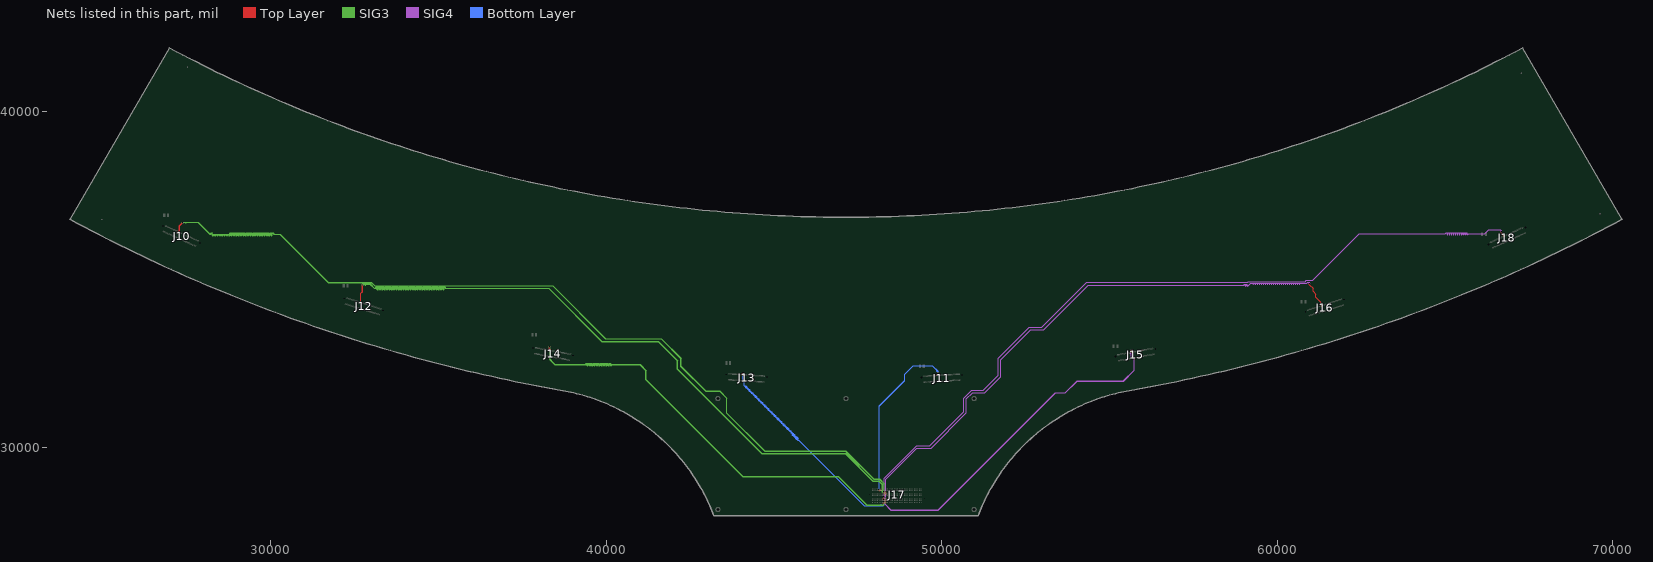
[diagram p0: the nets of this part, all layers, seen from the top]
# Altium PCB MISC86329.PcbDoc (part 8 of 11)
Units mil, origin at the board's own origin, x right, y up, seen from the top; angles counter-clockwise.
Board outline 46247.15 x 13937.21 mil, 6 copper layers (Top Layer, GND2, SIG3, SIG4, POWER5, Bottom Layer); 17 components, 210 nets, 908 pads, 1109 vias.

## Via types
v1: diameter 24, hole 12, Top Layer to Bottom Layer, 684 vias
v2: diameter 18, hole 9, Top Layer to Bottom Layer, 425 vias

## Nets (pads, with @x,y where several pads share a name; then routed paths per layer and width w, separated by ;. In a path a pad name is that pad's centre, name@x,y a point inside that pad or via, vN(x,y) a via of type N, cw(c..) or ccw(c..) an arc to the next point about the centre after c; other vN are vias at no path point) (continued)
DATAIN6N_CH0: J10.30 J17.G23 | length 28226.7
  Top Layer w5: J10.30@27279.03,36418.73 27279.03,36446.33 27291,36458.3 27291,36604 27383.75,36696.75 27386.6,36693.9 v2(27386.6,36690.4) ; v2(48264.09,28692.61) J17.G23@48287.89,28668.8
  SIG3 w5: v2@27383.75,36696.75 27398,36711 27462,36711 27467,36706 27467,36697.6 27472,36692.6 27482,36692.6 27487,36697.6 27487,36706 27492,36711 27838,36711 28196,36353 28223.82,36353 28235.5,36364.68 28235.5,36386.58 28241.32,36392.41 28254.68,36392.41 28260.5,36386.58 28260.5,36325.27 28272.18,36313.59 28293.82,36313.59 28305.5,36325.27 28305.5,36347.18 28311.32,36353 28324.68,36353 28330.5,36347.18 28330.5,36325.27 28342.18,36313.59 28363.82,36313.59 28375.5,36325.27 28375.5,36347.18 28381.32,36353 28394.68,36353 28400.5,36347.18 28400.5,36325.27 28412.18,36313.59 28433.82,36313.59 28445.5,36325.27 28445.5,36347.18 28451.32,36353 28464.68,36353 28470.5,36347.18 28470.5,36325.27 28482.18,36313.59 28503.82,36313.59 28515.5,36325.27 28515.5,36347.18 28521.32,36353 28534.68,36353 28540.5,36347.18 28540.5,36325.27 28552.18,36313.59 28573.82,36313.59 28585.5,36325.27 28585.5,36347.18 28591.32,36353 28604.68,36353 28610.5,36347.18 28610.5,36325.27 28622.18,36313.59 28643.82,36313.59 28655.5,36325.27 28655.5,36347.18 28661.32,36353 28674.68,36353 28680.5,36347.18 28680.5,36325.27 28692.18,36313.59 28713.82,36313.59 28725.5,36325.27 28725.5,36347.18 28731.32,36353 28744.68,36353 28750.5,36347.18 28750.5,36325.27 28762.18,36313.59 28783.82,36313.59 28795.5,36325.27 28795.5,36386.58 28801.32,36392.41 28814.68,36392.41 28820.5,36386.58 28820.5,36325.27 28832.18,36313.59 28853.82,36313.59 28865.5,36325.27 28865.5,36386.58 28871.32,36392.41 28884.68,36392.41 28890.5,36386.58 28890.5,36325.27 28902.18,36313.59 28923.82,36313.59 28935.5,36325.27 28935.5,36386.58 28941.32,36392.41 28954.68,36392.41 28960.5,36386.58 28960.5,36325.27 28972.18,36313.59 28993.82,36313.59 29005.5,36325.27 29005.5,36386.58 29011.32,36392.41 29024.68,36392.41 29030.5,36386.58 29030.5,36325.27 29042.18,36313.59 29063.82,36313.59 29075.5,36325.27 29075.5,36386.58 29081.32,36392.41 29094.68,36392.41 29100.5,36386.58 29100.5,36325.27 29112.18,36313.59 29133.82,36313.59 29145.5,36325.27 29145.5,36386.58 29151.32,36392.41 29164.68,36392.41 29170.5,36386.58 29170.5,36325.27 29182.18,36313.59 29203.82,36313.59 29215.5,36325.27 29215.5,36386.58 29221.32,36392.41 29234.68,36392.41 29240.5,36386.58 29240.5,36325.27 29252.18,36313.59 29273.82,36313.59 29285.5,36325.27 29285.5,36386.58 29291.32,36392.41 29304.68,36392.41 29310.5,36386.58 29310.5,36325.27 29322.18,36313.59 29343.82,36313.59 29355.5,36325.27 29355.5,36386.58 29361.32,36392.41 29374.68,36392.41 29380.5,36386.58 29380.5,36325.27 29392.18,36313.59 29413.82,36313.59 29425.5,36325.27 29425.5,36386.58 29431.32,36392.41 29444.68,36392.41 29450.5,36386.58 29450.5,36325.27 29462.18,36313.59 29483.82,36313.59 29495.5,36325.27 29495.5,36386.58 29501.32,36392.41 29514.68,36392.41 29520.5,36386.58 29520.5,36325.27 29532.18,36313.59 29553.82,36313.59 29565.5,36325.27 29565.5,36386.58 29571.32,36392.41 29584.68,36392.41 29590.5,36386.58 29590.5,36325.27 29602.18,36313.59 29623.82,36313.59 29635.5,36325.27 29635.5,36386.58 29641.32,36392.41 29654.68,36392.41 29660.5,36386.58 29660.5,36325.27 29672.18,36313.59 29693.82,36313.59 29705.5,36325.27 29705.5,36386.58 29711.32,36392.41 29724.68,36392.41 29730.5,36386.58 29730.5,36325.27 29742.18,36313.59 29763.82,36313.59 29775.5,36325.27 29775.5,36386.58 29781.32,36392.41 29794.68,36392.41 29800.5,36386.58 29800.5,36325.27 29812.18,36313.59 29833.82,36313.59 29845.5,36325.27 29845.5,36386.58 29851.32,36392.41 29864.68,36392.41 29870.5,36386.58 29870.5,36325.27 29882.18,36313.59 29903.82,36313.59 29915.5,36325.27 29915.5,36386.58 29921.32,36392.41 29934.68,36392.41 29940.5,36386.58 29940.5,36325.27 29952.18,36313.59 29973.82,36313.59 29985.5,36325.27 29985.5,36386.58 29991.32,36392.41 30004.68,36392.41 30010.5,36386.58 30010.5,36325.27 30022.18,36313.59 30043.82,36313.59 30055.5,36325.27 30055.5,36386.58 30061.32,36392.41 30074.68,36392.41 30080.5,36386.58 30080.5,36364.68 30092.18,36353 30281.86,36353 31717.86,34917 33003.86,34917 33104.86,34816 38404.86,34816 39981.86,33239 41642,33239 42230,32651 42230,32414.86 42966.86,31678 43382.86,31678 43592,31468.86 43592,31025.86 44721.86,29896 47133.86,29896 47970.86,29059 48145.86,29059 48284.09,28920.77 48284.09,28712.61 v2(48264.09,28692.61)
DATAIN6N_CH1: J12.30 J17.F23 | length 23094.8
  Top Layer w5: J12.30@32696.65,34319.49 32696,34320.14 32696,34596 32745,34645 32745,34837.5 v2(32751.5,34844) ; v2(48264.09,28642.61) J17.F23@48287.89,28618.8
  SIG3 w5: v2(32751.5,34844) 32745,34850.5 32745,34857.86 32756.14,34869 32783,34869 32795.5,34869 32814.25,34869 32820.5,34862.75 32820.5,34838.79 32826.75,34832.54 32839.25,34832.54 32845.5,34838.79 32845.5,34862.75 32851.75,34869 32962,34869 32970.84,34860.16 ; 32964.5,34866.5 33089,34742 33134.82,34742 33146.5,34753.68 33146.5,34775.69 33152.32,34781.52 33165.68,34781.52 33171.5,34775.69 33171.5,34714.16 33183.18,34702.48 33204.82,34702.48 33216.5,34714.16 33216.5,34775.69 33222.32,34781.52 33235.68,34781.52 33241.5,34775.69 33241.5,34714.16 33253.18,34702.48 33274.82,34702.48 33286.5,34714.16 33286.5,34775.69 33292.32,34781.52 33305.68,34781.52 33311.5,34775.69 33311.5,34714.16 33323.18,34702.48 33344.82,34702.48 33356.5,34714.16 33356.5,34775.69 33362.32,34781.52 33375.68,34781.52 33381.5,34775.69 33381.5,34714.16 33393.18,34702.48 33414.82,34702.48 33426.5,34714.16 33426.5,34775.69 33432.32,34781.52 33445.68,34781.52 33451.5,34775.69 33451.5,34714.16 33463.18,34702.48 33484.82,34702.48 33496.5,34714.16 33496.5,34775.69 33502.32,34781.52 33515.68,34781.52 33521.5,34775.69 33521.5,34714.16 33533.18,34702.48 33554.82,34702.48 33566.5,34714.16 33566.5,34775.69 33572.32,34781.52 33585.68,34781.52 33591.5,34775.69 33591.5,34714.16 33603.18,34702.48 33624.82,34702.48 33636.5,34714.16 33636.5,34775.69 33642.32,34781.52 33655.68,34781.52 33661.5,34775.69 33661.5,34714.16 33673.18,34702.48 33694.82,34702.48 33706.5,34714.16 33706.5,34775.69 33712.32,34781.52 33725.68,34781.52 33731.5,34775.69 33731.5,34714.16 33743.18,34702.48 33764.82,34702.48 33776.5,34714.16 33776.5,34775.69 33782.32,34781.52 33795.68,34781.52 33801.5,34775.69 33801.5,34714.16 33813.18,34702.48 33834.82,34702.48 33846.5,34714.16 33846.5,34775.69 33852.32,34781.52 33865.68,34781.52 33871.5,34775.69 33871.5,34714.16 33883.18,34702.48 33904.82,34702.48 33916.5,34714.16 33916.5,34775.69 33922.32,34781.52 33935.68,34781.52 33941.5,34775.69 33941.5,34714.16 33953.18,34702.48 33974.82,34702.48 33986.5,34714.16 33986.5,34775.69 33992.32,34781.52 34005.68,34781.52 34011.5,34775.69 34011.5,34714.16 34023.18,34702.48 34044.82,34702.48 34056.5,34714.16 34056.5,34775.69 34062.32,34781.52 34075.68,34781.52 34081.5,34775.69 34081.5,34714.16 34093.18,34702.48 34114.82,34702.48 34126.5,34714.16 34126.5,34775.69 34132.32,34781.52 34145.68,34781.52 34151.5,34775.69 34151.5,34714.16 34163.18,34702.48 34184.82,34702.48 34196.5,34714.16 34196.5,34775.69 34202.32,34781.52 34215.68,34781.52 34221.5,34775.69 34221.5,34714.16 34233.18,34702.48 34254.82,34702.48 34266.5,34714.16 34266.5,34775.69 34272.32,34781.52 34285.68,34781.52 34291.5,34775.69 34291.5,34714.16 34303.18,34702.48 34324.82,34702.48 34336.5,34714.16 34336.5,34775.69 34342.32,34781.52 34355.68,34781.52 34361.5,34775.69 34361.5,34714.16 34373.18,34702.48 34394.82,34702.48 34406.5,34714.16 34406.5,34775.69 34412.32,34781.52 34425.68,34781.52 34431.5,34775.69 34431.5,34714.16 34443.18,34702.48 34464.82,34702.48 34476.5,34714.16 34476.5,34775.69 34482.32,34781.52 34495.68,34781.52 34501.5,34775.69 34501.5,34714.16 34513.18,34702.48 34534.82,34702.48 34546.5,34714.16 34546.5,34775.69 34552.32,34781.52 34565.68,34781.52 34571.5,34775.69 34571.5,34714.16 34583.18,34702.48 34604.82,34702.48 34616.5,34714.16 34616.5,34775.69 34622.32,34781.52 34635.68,34781.52 34641.5,34775.69 34641.5,34714.16 34653.18,34702.48 34674.82,34702.48 34686.5,34714.16 34686.5,34775.69 34692.32,34781.52 34705.68,34781.52 34711.5,34775.69 34711.5,34714.16 34723.18,34702.48 34744.82,34702.48 34756.5,34714.16 34756.5,34775.69 34762.32,34781.52 34775.68,34781.52 34781.5,34775.69 34781.5,34714.16 34793.18,34702.48 34814.82,34702.48 34826.5,34714.16 34826.5,34775.69 34832.32,34781.52 34845.68,34781.52 34851.5,34775.69 34851.5,34714.16 34863.18,34702.48 34884.82,34702.48 34896.5,34714.16 34896.5,34775.69 34902.32,34781.52 34915.68,34781.52 34921.5,34775.69 34921.5,34714.16 34933.18,34702.48 34954.82,34702.48 34966.5,34714.16 34966.5,34775.69 34972.32,34781.52 34985.68,34781.52 34991.5,34775.69 34991.5,34714.16 35003.18,34702.48 35024.82,34702.48 35036.5,34714.16 35036.5,34775.69 35042.32,34781.52 35055.68,34781.52 35061.5,34775.69 35061.5,34714.16 35073.18,34702.48 35094.82,34702.48 35106.5,34714.16 35106.5,34775.69 35112.32,34781.52 35125.68,34781.52 35131.5,34775.69 35131.5,34714.16 35143.18,34702.48 35164.82,34702.48 35176.5,34714.16 35176.5,34775.69 35182.32,34781.52 35195.68,34781.52 35201.5,34775.69 35201.5,34753.68 35213.18,34742 38287.86,34742 39873.86,33156 41550,33156 42119,32587 42119,32333.86 44637.86,29815 47132.86,29815 47944.86,29003 48126.86,29003 48233,28896.86 48233,28676 48256.96,28652.04 48264.09,28644.91 v2(48264.09,28642.61)
DATAIN6N_CH2: J14.30 J17.B23 | length 13805.7
  Top Layer w5: v2(38324.5,33005) 38318,32998.5 38318,32928 38329.73,32916.27 J14.30@38329.73,32896.14 ; v2(48264.09,28395) J17.B23@48287.89,28418.8
  SIG3 w5: v2@38322,33002 38317,32997 38317,32962.14 38330,32949.14 38330,32898.75 38336.25,32892.5 38343.96,32892.5 38350.21,32886.25 38350.21,32873.75 38343.96,32867.5 38336.25,32867.5 38330,32861.25 38330,32629 38347.49,32611.51 38361.25,32597.75 38381.81,32577.19 38476,32483 39384.68,32483 39390.5,32488.82 39390.5,32501.32 39402.18,32513 39423.82,32513 39435.5,32501.32 39435.5,32451.39 39441.32,32445.57 39454.68,32445.57 39460.5,32451.39 39460.5,32501.32 39472.18,32513 39493.82,32513 39505.5,32501.32 39505.5,32451.39 39511.32,32445.57 39524.68,32445.57 39530.5,32451.39 39530.5,32501.32 39542.18,32513 39563.82,32513 39575.5,32501.32 39575.5,32451.39 39581.32,32445.57 39594.68,32445.57 39600.5,32451.39 39600.5,32501.32 39612.18,32513 39633.82,32513 39645.5,32501.32 39645.5,32451.39 39651.32,32445.57 39664.68,32445.57 39670.5,32451.39 39670.5,32501.32 39682.18,32513 39703.82,32513 39715.5,32501.32 39715.5,32451.39 39721.32,32445.57 39734.68,32445.57 39740.5,32451.39 39740.5,32501.32 39752.18,32513 39773.82,32513 39785.5,32501.32 39785.5,32451.39 39791.32,32445.57 39804.68,32445.57 39810.5,32451.39 39810.5,32501.32 39822.18,32513 39843.82,32513 39855.5,32501.32 39855.5,32451.39 39861.32,32445.57 39874.68,32445.57 39880.5,32451.39 39880.5,32501.32 39892.18,32513 39913.82,32513 39925.5,32501.32 39925.5,32451.39 39931.32,32445.57 39944.68,32445.57 39950.5,32451.39 39950.5,32501.32 39962.18,32513 39983.82,32513 39995.5,32501.32 39995.5,32451.39 40001.32,32445.57 40014.68,32445.57 40020.5,32451.39 40020.5,32501.32 40032.18,32513 40053.82,32513 40065.5,32501.32 40065.5,32451.39 40071.32,32445.57 40084.68,32445.57 40090.5,32451.39 40090.5,32501.32 40102.18,32513 40123.82,32513 40135.5,32501.32 40135.5,32451.39 40141.32,32445.57 40154.68,32445.57 40160.5,32451.39 40160.5,32471.32 40172.18,32483 41011,32483 41199,32295 41199,32024 44075,29148 46915,29148 47770,28293 48253,28293 48285,28325 48285,28374.09 v2(48264.09,28395)
DATAIN6N_CH3: J13.30 J17.A23 | length 7746.4
  Top Layer w5: 44083.13,32206.15 44094.28,32195 J13.30@44094.28,32169.89 ; 44083.56,32206.58 44083.56,32233.5 ; v2(48264.09,28345) J17.A23@48287.89,28368.8
  Bottom Layer w5: 44084,32223 44084,32222 ; v2(44090.06,32240) 44084,32233.94 44084,32222 ; v2(48264.09,28345) 48284.09,28325 48284.09,28300 48254.09,28270 48213.82,28270 48210.5,28273.32 48210.5,28280.82 48201.32,28290 48184.68,28290 48175.5,28280.82 48175.5,28273.32 48172.18,28270 47699.14,28270 45732.97,30236.17 45721.76,30236.17 45714.69,30229.1 45711.76,30229.1 45704.08,30236.78 45704.08,30239.71 45725.29,30260.92 45725.29,30272.13 45711.76,30285.67 45700.54,30285.67 45679.33,30264.46 45676.4,30264.46 45668.72,30272.13 45668.72,30275.06 45689.94,30296.27 45689.94,30307.49 45676.4,30321.02 45665.19,30321.02 45643.98,30299.81 45641.05,30299.81 45633.37,30307.49 45633.37,30310.42 45654.58,30331.63 45654.58,30342.84 45641.05,30356.38 45629.83,30356.38 45608.62,30335.17 45605.69,30335.17 45598.01,30342.84 45598.01,30345.77 45619.23,30366.99 45619.23,30378.2 45605.69,30391.73 45594.48,30391.73 45573.27,30370.52 45570.34,30370.52 45562.66,30378.2 45562.66,30381.13 45583.87,30402.34 45583.87,30413.55 45570.34,30427.09 45559.12,30427.09 45552.05,30420.02 45549.12,30420.02 45541.45,30427.7 45541.45,30430.63 45548.52,30437.7 45548.52,30448.91 45534.98,30462.44 45523.77,30462.44 45516.7,30455.37 45513.77,30455.37 45506.09,30463.05 45506.09,30465.98 45513.16,30473.05 45513.16,30484.26 45499.63,30497.8 45488.41,30497.8 45481.34,30490.73 45478.41,30490.73 45470.74,30498.41 45470.74,30501.34 45477.81,30508.41 45477.81,30519.62 45464.27,30533.16 45453.06,30533.16 45445.99,30526.08 45443.06,30526.08 45435.38,30533.76 45435.38,30536.69 45442.45,30543.76 45442.45,30554.98 45428.92,30568.51 45417.7,30568.51 45410.63,30561.44 45407.7,30561.44 45400.02,30569.12 45400.02,30572.05 45407.1,30579.12 45407.1,30590.33 45393.56,30603.87 45382.35,30603.87 45375.28,30596.8 45372.35,30596.8 45364.67,30604.47 45364.67,30607.4 45371.74,30614.47 45371.74,30625.69 45358.2,30639.22 45346.99,30639.22 45339.92,30632.15 45336.99,30632.15 45329.31,30639.83 45329.31,30642.76 45336.38,30649.83 45336.38,30661.04 45322.85,30674.58 45311.64,30674.58 45304.56,30667.51 45301.64,30667.51 45293.96,30675.18 45293.96,30678.11 45301.03,30685.18 45301.03,30696.4 45287.49,30709.93 45276.28,30709.93 45269.21,30702.86 45266.28,30702.86 45258.6,30710.54 45258.6,30713.47 45265.67,30720.54 45265.67,30731.75 45252.14,30745.29 45240.93,30745.29 45233.85,30738.22 45230.93,30738.22 45223.25,30745.89 45223.25,30748.82 45230.32,30755.89 45230.32,30767.11 45216.78,30780.64 45205.57,30780.64 45198.5,30773.57 45195.57,30773.57 45187.89,30781.25 45187.89,30784.18 45194.96,30791.25 45194.96,30802.46 45181.43,30816 45170.21,30816 45163.14,30808.93 45160.21,30808.93 45152.54,30816.6 45152.54,30819.53 45159.61,30826.6 45159.61,30837.82 45146.07,30851.35 45134.86,30851.35 45127.79,30844.28 45124.86,30844.28 45117.18,30851.96 45117.18,30854.89 45124.25,30861.96 45124.25,30873.17 45110.72,30886.71 45099.5,30886.71 45092.43,30879.64 45089.5,30879.64 45081.83,30887.32 45081.83,30890.24 45088.9,30897.32 45088.9,30908.53 45075.36,30922.06 45064.15,30922.06 45057.08,30914.99 45054.15,30914.99 45046.47,30922.67 45046.47,30925.6 45053.54,30932.67 45053.54,30943.88 45040.01,30957.42 45028.79,30957.42 45021.72,30950.35 45018.79,30950.35 45011.12,30958.03 45011.12,30960.96 45018.19,30968.03 45018.19,30979.24 45004.65,30992.78 44993.44,30992.78 44986.37,30985.7 44983.44,30985.7 44975.76,30993.38 44975.76,30996.31 44982.83,31003.38 44982.83,31014.6 44969.3,31028.13 44958.08,31028.13 44951.01,31021.06 44948.08,31021.06 44940.4,31028.74 44940.4,31031.67 44947.48,31038.74 44947.48,31049.95 44933.94,31063.49 44922.73,31063.49 44915.66,31056.41 44912.73,31056.41 44905.05,31064.09 44905.05,31067.02 44912.12,31074.09 44912.12,31085.31 44898.59,31098.84 44887.37,31098.84 44880.3,31091.77 44877.37,31091.77 44869.69,31099.45 44869.69,31102.38 44876.77,31109.45 44876.77,31120.66 44863.23,31134.2 44852.02,31134.2 44844.95,31127.13 44842.02,31127.13 44834.34,31134.8 44834.34,31137.73 44841.41,31144.8 44841.41,31156.02 44827.87,31169.55 44816.66,31169.55 44809.59,31162.48 44806.66,31162.48 44798.98,31170.16 44798.98,31173.09 44806.05,31180.16 44806.05,31191.37 44792.52,31204.91 44781.31,31204.91 44774.23,31197.84 44771.31,31197.84 44763.63,31205.51 44763.63,31208.44 44770.7,31215.51 44770.7,31226.73 44757.16,31240.26 44745.95,31240.26 44738.88,31233.19 44735.95,31233.19 44728.27,31240.87 44728.27,31243.8 44735.34,31250.87 44735.34,31262.08 44721.81,31275.62 44710.6,31275.62 44703.52,31268.55 44700.6,31268.55 44692.92,31276.22 44692.92,31279.15 44699.99,31286.22 44699.99,31297.44 44686.45,31310.97 44675.24,31310.97 44668.17,31303.9 44665.24,31303.9 44657.56,31311.58 44657.56,31314.51 44664.63,31321.58 44664.63,31332.79 44651.1,31346.33 44639.88,31346.33 44632.81,31339.26 44629.88,31339.26 44622.21,31346.94 44622.21,31349.86 44629.28,31356.94 44629.28,31368.15 44615.74,31381.68 44604.53,31381.68 44597.46,31374.61 44594.53,31374.61 44586.85,31382.29 44586.85,31385.22 44593.92,31392.29 44593.92,31403.5 44580.39,31417.04 44569.17,31417.04 44562.1,31409.97 44559.17,31409.97 44551.5,31417.65 44551.5,31420.57 44558.57,31427.65 44558.57,31438.86 44545.03,31452.39 44533.82,31452.39 44526.75,31445.32 44523.82,31445.32 44516.14,31453 44516.14,31455.93 44523.21,31463 44523.21,31474.21 44509.68,31487.75 44498.46,31487.75 44491.39,31480.68 44488.46,31480.68 44480.79,31488.36 44480.79,31491.29 44487.86,31498.36 44487.86,31509.57 44474.32,31523.11 44463.11,31523.11 44456.04,31516.03 44453.11,31516.03 44445.43,31523.71 44445.43,31526.64 44452.5,31533.71 44452.5,31544.93 44438.97,31558.46 44427.75,31558.46 44420.68,31551.39 44417.75,31551.39 44410.07,31559.07 44410.07,31562 44417.15,31569.07 44417.15,31580.28 44403.61,31593.82 44392.4,31593.82 44385.33,31586.74 44382.4,31586.74 44374.72,31594.42 44374.72,31597.35 44381.79,31604.42 44381.79,31615.64 44368.26,31629.17 44357.04,31629.17 44349.97,31622.1 44347.04,31622.1 44339.36,31629.78 44339.36,31632.71 44346.44,31639.78 44346.44,31650.99 44332.9,31664.53 44321.69,31664.53 44314.62,31657.46 44311.69,31657.46 44304.01,31665.13 44304.01,31668.06 44311.08,31675.13 44311.08,31686.35 44297.54,31699.88 44286.33,31699.88 44279.26,31692.81 44276.33,31692.81 44268.65,31700.49 44268.65,31703.42 44275.72,31710.49 44275.72,31721.7 44262.19,31735.24 44250.98,31735.24 44243.9,31728.17 44240.98,31728.17 44233.3,31735.84 44233.3,31738.77 44240.37,31745.84 44240.37,31757.06 44226.83,31770.59 44215.62,31770.59 44208.55,31763.52 44205.62,31763.52 44197.94,31771.2 44197.94,31774.13 44205.01,31781.2 44205.01,31792.41 44191.48,31805.95 44180.27,31805.95 44173.19,31798.88 44170.27,31798.88 44162.59,31806.55 44162.59,31809.48 44169.66,31816.55 44169.66,31827.77 44156.12,31841.3 44144.91,31841.3 44137.84,31834.23 44134.91,31834.23 44121,31848.14 44121,31973 44084,32010 44084,32155.25 44090.25,32161.5 44100.57,32161.5 44106.82,32167.75 44106.82,32180.25 44100.57,32186.5 44090.25,32186.5 44084,32192.75 44084,32222
DATAIN6N_CH4: J11.30 J17.H26 | length 5094.9
  Top Layer w5: v2(48114.09,28742.61) J17.H26@48137.89,28718.8 ; 49893.65,32207.5 49893.65,32187.72 49904.37,32177 J11.30@49904.37,32151.58
  Bottom Layer w5: v2(48114.09,28742.61) 48134.09,28762.61 48134.09,31240.09 48893,31999 48893,32183 49151,32441 49724.14,32441 49894,32271.14 49894,32243 ; 49894,32234.63 49894,32243 ; 49894,32235 49894,32221 v2@49899,32216 ; 49894,32241 49894,32243
  other v2: 49900.15,32214
DATAIN6N_CH5: J15.30 J17.C23 | length 10126.4
  Top Layer w5: v2(48264.09,28445) J17.C23@48287.89,28468.8 ; 55656,32901.5 55656,32885.39 55673.39,32868 J15.30@55673.39,32841.48
  SIG4 w5: v2(48264.09,28445) 48284.09,28425 48284.09,28333.91 48483,28135 49902.14,28135 53394.14,31627 53681.14,31627 54037.14,31983 55418.14,31983 55742,32306.86 55742,32629.14 55656,32715.14 55656,32835 55656,32902 v2@55661,32907
  other v2: 55662.5,32908
DATAIN6N_CH6: J16.30 J17.D23 | length 18290.6
  Top Layer w5: v2(48264.09,28495) J17.D23@48287.89,28518.8 ; 60959,34880.5 60959,34850.14 61065,34744.14 61065,34652.14 61151,34566.14 61151,34478.14 61296,34333.14 61296,34252 61315.32,34232.68 J16.30@61315.32,34229.3
  SIG4 w5: v2(48264.09,28495) 48290.75,28495 48307.25,28511.5 48316.44,28511.5 48334,28529.06 48334,29057.14 49263.86,29987 49693,29987 50737,31031 50737,31450.14 50923.86,31637 51281,31637 51754,32110 51754,32616.14 52648.86,33511 53042,33511 54373,34842 59005,34842 59009.57,34846.57 59009.57,34861.57 59020,34872 59039.14,34872 59049.57,34861.57 59049.57,34816.57 59054.14,34812 59065,34812 59069.57,34816.57 59069.57,34861.57 59080,34872 59099.14,34872 59109.57,34861.57 59109.57,34816.57 59114.14,34812 59125,34812 59129.57,34816.57 59129.57,34831.57 59140,34842 59155,34842 59214,34901 59265.07,34901 59275.5,34890.57 59275.5,34875.57 59280.07,34871 59290.93,34871 59295.5,34875.57 59295.5,34890.57 59305.93,34901 59325.07,34901 59335.5,34890.57 59335.5,34875.57 59340.07,34871 59350.93,34871 59355.5,34875.57 59355.5,34890.57 59365.93,34901 59385.07,34901 59395.5,34890.57 59395.5,34875.57 59400.07,34871 59410.93,34871 59415.5,34875.57 59415.5,34890.57 59425.93,34901 59445.07,34901 59455.5,34890.57 59455.5,34875.57 59460.07,34871 59470.93,34871 59475.5,34875.57 59475.5,34890.57 59485.93,34901 59505.07,34901 59515.5,34890.57 59515.5,34875.57 59520.07,34871 59530.93,34871 59535.5,34875.57 59535.5,34890.57 59545.93,34901 59565.07,34901 59575.5,34890.57 59575.5,34875.57 59580.07,34871 59590.93,34871 59595.5,34875.57 59595.5,34890.57 59605.93,34901 59625.07,34901 59635.5,34890.57 59635.5,34875.57 59640.07,34871 59650.93,34871 59655.5,34875.57 59655.5,34890.57 59665.93,34901 59685.07,34901 59695.5,34890.57 59695.5,34875.57 59700.07,34871 59710.93,34871 59715.5,34875.57 59715.5,34890.57 59725.93,34901 59745.07,34901 59755.5,34890.57 59755.5,34875.57 59760.07,34871 59770.93,34871 59775.5,34875.57 59775.5,34890.57 59785.93,34901 59805.07,34901 59815.5,34890.57 59815.5,34875.57 59820.07,34871 59830.93,34871 59835.5,34875.57 59835.5,34890.57 59845.93,34901 59865.07,34901 59875.5,34890.57 59875.5,34875.57 59880.07,34871 59890.93,34871 59895.5,34875.57 59895.5,34890.57 59905.93,34901 59925.07,34901 59935.5,34890.57 59935.5,34875.57 59940.07,34871 59950.93,34871 59955.5,34875.57 59955.5,34890.57 59965.93,34901 59985.07,34901 59995.5,34890.57 59995.5,34875.57 60000.07,34871 60010.93,34871 60015.5,34875.57 60015.5,34890.57 60025.93,34901 60045.07,34901 60055.5,34890.57 60055.5,34875.57 60060.07,34871 60070.93,34871 60075.5,34875.57 60075.5,34890.57 60085.93,34901 60105.07,34901 60115.5,34890.57 60115.5,34875.57 60120.07,34871 60130.93,34871 60135.5,34875.57 60135.5,34890.57 60145.93,34901 60165.07,34901 60175.5,34890.57 60175.5,34875.57 60180.07,34871 60190.93,34871 60195.5,34875.57 60195.5,34890.57 60205.93,34901 60225.07,34901 60235.5,34890.57 60235.5,34875.57 60240.07,34871 60250.93,34871 60255.5,34875.57 60255.5,34890.57 60265.93,34901 60285.07,34901 60295.5,34890.57 60295.5,34875.57 60300.07,34871 60310.93,34871 60315.5,34875.57 60315.5,34890.57 60325.93,34901 60345.07,34901 60355.5,34890.57 60355.5,34875.57 60360.07,34871 60370.93,34871 60375.5,34875.57 60375.5,34890.57 60385.93,34901 60405.07,34901 60415.5,34890.57 60415.5,34875.57 60420.07,34871 60430.93,34871 60435.5,34875.57 60435.5,34890.57 60445.93,34901 60465.07,34901 60475.5,34890.57 60475.5,34875.57 60480.07,34871 60490.93,34871 60495.5,34875.57 60495.5,34890.57 60505.93,34901 60525.07,34901 60535.5,34890.57 60535.5,34875.57 60540.07,34871 60550.93,34871 60555.5,34875.57 60555.5,34890.57 60565.93,34901 60585.07,34901 60595.5,34890.57 60595.5,34875.57 60600.07,34871 60610.93,34871 60615.5,34875.57 60615.5,34890.57 60625.93,34901 60645.07,34901 60655.5,34890.57 60655.5,34875.57 60660.07,34871 60670.93,34871 60675.5,34875.57 60675.5,34890.57 60685.93,34901 60703,34901 60791,34901 60821,34901 60831,34901 60878,34901 60904,34927 60945.14,34927 60959,34913.14 60959,34894 v2@60965,34888
  other v2: 60965.5,34887
DATAIN6N_CH7: J17.E23 J18.30 | length 23893.4
  Top Layer w5: v2(48264.09,28545) J17.E23@48287.89,28568.8 ; v2(66681.5,36430) 66675,36423.5 66675,36394.14 66727.39,36341.75 66727.39,36313.04 J18.30@66746.07,36294.36
  SIG4 w5: v2(48264.09,28545) 48284.09,28565 48284.09,29085.23 49255.86,30057 49651,30057 50659,31065 50659,31469 50891,31701 51232,31701 51688,32157 51688,32660.14 52613.86,33586 52986,33586 54324,34924 59113,34924 59133,34944 60826,34944 60864,34982 61053,34982 62448,36377 65003.86,36377 65033.86,36407 65053.57,36407 65064,36396.57 65064,36351.57 65068.57,36347 65079.43,36347 65084,36351.57 65084,36396.57 65094.43,36407 65113.57,36407 65124,36396.57 65124,36351.57 65128.57,36347 65139.43,36347 65144,36351.57 65144,36396.57 65154.43,36407 65173.57,36407 65184,36396.57 65184,36351.57 65188.57,36347 65199.43,36347 65204,36351.57 65204,36396.57 65214.43,36407 65233.57,36407 65244,36396.57 65244,36351.57 65248.57,36347 65259.43,36347 65264,36351.57 65264,36396.57 65274.43,36407 65293.57,36407 65304,36396.57 65304,36351.57 65308.57,36347 65319.43,36347 65324,36351.57 65324,36396.57 65334.43,36407 65353.57,36407 65364,36396.57 65364,36351.57 65368.57,36347 65379.43,36347 65384,36351.57 65384,36396.57 65394.43,36407 65413.57,36407 65424,36396.57 65424,36351.57 65428.57,36347 65439.43,36347 65444,36351.57 65444,36396.57 65454.43,36407 65473.57,36407 65484,36396.57 65484,36351.57 65488.57,36347 65499.43,36347 65504,36351.57 65504,36396.57 65514.43,36407 65533.57,36407 65544,36396.57 65544,36351.57 65548.57,36347 65559.43,36347 65564,36351.57 65564,36396.57 65574.43,36407 65593.57,36407 65604,36396.57 65604,36351.57 65608.57,36347 65619.43,36347 65624,36351.57 65624,36396.57 65634.43,36407 65653.57,36407 65664,36396.57 65664,36351.57 65668.57,36347 65679.43,36347 65684,36351.57 65684,36366.57 65694.43,36377 66185,36377 66300,36492 66641.14,36492 66675,36458.14 66675,36438 v2@66682,36431
DATAIN6P_CH0: J10.28 J17.G22 | length 28227.3
  Top Layer w5: J10.28@27250.38,36431.83 27281,36462.45 27281,36608.14 27370.33,36697.47 v2(27370.33,36706.67) ; v2(48314.09,28692.61) J17.G22@48337.89,28668.8
  SIG3 w5: v2(27370.33,36706.67) 27379.53,36706.67 27393.86,36721 27462,36721 27842.14,36721 28200.14,36363 28219.68,36363 28225.5,36368.82 28225.5,36390.73 28237.18,36402.41 28258.82,36402.41 28270.5,36390.73 28270.5,36329.42 28276.32,36323.59 28289.68,36323.59 28295.5,36329.42 28295.5,36351.32 28307.18,36363 28328.82,36363 28340.5,36351.32 28340.5,36329.42 28346.32,36323.59 28359.68,36323.59 28365.5,36329.42 28365.5,36351.32 28377.18,36363 28398.82,36363 28410.5,36351.32 28410.5,36329.42 28416.32,36323.59 28429.68,36323.59 28435.5,36329.42 28435.5,36351.32 28447.18,36363 28468.82,36363 28480.5,36351.32 28480.5,36329.42 28486.32,36323.59 28499.68,36323.59 28505.5,36329.42 28505.5,36351.32 28517.18,36363 28538.82,36363 28550.5,36351.32 28550.5,36329.42 28556.32,36323.59 28569.68,36323.59 28575.5,36329.42 28575.5,36351.32 28587.18,36363 28608.82,36363 28620.5,36351.32 28620.5,36329.42 28626.32,36323.59 28639.68,36323.59 28645.5,36329.42 28645.5,36351.32 28657.18,36363 28678.82,36363 28690.5,36351.32 28690.5,36329.42 28696.32,36323.59 28709.68,36323.59 28715.5,36329.42 28715.5,36351.32 28727.18,36363 28748.82,36363 28760.5,36351.32 28760.5,36329.42 28766.32,36323.59 28779.68,36323.59 28785.5,36329.42 28785.5,36390.73 28797.18,36402.41 28818.82,36402.41 28830.5,36390.73 28830.5,36329.42 28836.32,36323.59 28849.68,36323.59 28855.5,36329.42 28855.5,36390.73 28867.18,36402.41 28888.82,36402.41 28900.5,36390.73 28900.5,36329.42 28906.32,36323.59 28919.68,36323.59 28925.5,36329.42 28925.5,36390.73 28937.18,36402.41 28958.82,36402.41 28970.5,36390.73 28970.5,36329.42 28976.32,36323.59 28989.68,36323.59 28995.5,36329.42 28995.5,36390.73 29007.18,36402.41 29028.82,36402.41 29040.5,36390.73 29040.5,36329.42 29046.32,36323.59 29059.68,36323.59 29065.5,36329.42 29065.5,36390.73 29077.18,36402.41 29098.82,36402.41 29110.5,36390.73 29110.5,36329.42 29116.32,36323.59 29129.68,36323.59 29135.5,36329.42 29135.5,36390.73 29147.18,36402.41 29168.82,36402.41 29180.5,36390.73 29180.5,36329.42 29186.32,36323.59 29199.68,36323.59 29205.5,36329.42 29205.5,36390.73 29217.18,36402.41 29238.82,36402.41 29250.5,36390.73 29250.5,36329.42 29256.32,36323.59 29269.68,36323.59 29275.5,36329.42 29275.5,36390.73 29287.18,36402.41 29308.82,36402.41 29320.5,36390.73 29320.5,36329.42 29326.32,36323.59 29339.68,36323.59 29345.5,36329.42 29345.5,36390.73 29357.18,36402.41 29378.82,36402.41 29390.5,36390.73 29390.5,36329.42 29396.32,36323.59 29409.68,36323.59 29415.5,36329.42 29415.5,36390.73 29427.18,36402.41 29448.82,36402.41 29460.5,36390.73 29460.5,36329.42 29466.32,36323.59 29479.68,36323.59 29485.5,36329.42 29485.5,36390.73 29497.18,36402.41 29518.82,36402.41 29530.5,36390.73 29530.5,36329.42 29536.32,36323.59 29549.68,36323.59 29555.5,36329.42 29555.5,36390.73 29567.18,36402.41 29588.82,36402.41 29600.5,36390.73 29600.5,36329.42 29606.32,36323.59 29619.68,36323.59 29625.5,36329.42 29625.5,36390.73 29637.18,36402.41 29658.82,36402.41 29670.5,36390.73 29670.5,36329.42 29676.32,36323.59 29689.68,36323.59 29695.5,36329.42 29695.5,36390.73 29707.18,36402.41 29728.82,36402.41 29740.5,36390.73 29740.5,36329.42 29746.32,36323.59 29759.68,36323.59 29765.5,36329.42 29765.5,36390.73 29777.18,36402.41 29798.82,36402.41 29810.5,36390.73 29810.5,36329.42 29816.32,36323.59 29829.68,36323.59 29835.5,36329.42 29835.5,36390.73 29847.18,36402.41 29868.82,36402.41 29880.5,36390.73 29880.5,36329.42 29886.32,36323.59 29899.68,36323.59 29905.5,36329.42 29905.5,36390.73 29917.18,36402.41 29938.82,36402.41 29950.5,36390.73 29950.5,36329.42 29956.32,36323.59 29969.68,36323.59 29975.5,36329.42 29975.5,36390.73 29987.18,36402.41 30008.82,36402.41 30020.5,36390.73 30020.5,36329.42 30026.32,36323.59 30039.68,36323.59 30045.5,36329.42 30045.5,36390.73 30057.18,36402.41 30078.82,36402.41 30090.5,36390.73 30090.5,36368.82 30096.32,36363 30286,36363 31722,34927 33008,34927 33109,34826 38409,34826 39986,33249 41646.14,33249 42240,32655.14 42240,32419 42971,31688 43387,31688 43602,31473 43602,31030 44726,29906 47138,29906 47975,29069 48150,29069 48294.09,28924.91 48294.09,28712.61 v2(48314.09,28692.61)
DATAIN6P_CH1: J12.28 J17.F22 | length 23095.2
  Top Layer w5: J12.28@32666.63,34329 32686,34348.37 32686,34600.14 32735,34649.14 32735,34837.5 v2(32728.5,34844) ; v2(48314.09,28642.61) J17.F22@48337.89,28618.8
  SIG3 w5: v2(32728.5,34844) 32735,34850.5 32735,34862 32752,34879 32966.14,34879 33093.14,34752 33130.68,34752 33136.5,34757.82 33136.5,34779.84 33148.18,34791.52 33169.82,34791.52 33181.5,34779.84 33181.5,34718.31 33187.32,34712.48 33200.68,34712.48 33206.5,34718.31 33206.5,34779.84 33218.18,34791.52 33239.82,34791.52 33251.5,34779.84 33251.5,34718.31 33257.32,34712.48 33270.68,34712.48 33276.5,34718.31 33276.5,34779.84 33288.18,34791.52 33309.82,34791.52 33321.5,34779.84 33321.5,34718.31 33327.32,34712.48 33340.68,34712.48 33346.5,34718.31 33346.5,34779.84 33358.18,34791.52 33379.82,34791.52 33391.5,34779.84 33391.5,34718.31 33397.32,34712.48 33410.68,34712.48 33416.5,34718.31 33416.5,34779.84 33428.18,34791.52 33449.82,34791.52 33461.5,34779.84 33461.5,34718.31 33467.32,34712.48 33480.68,34712.48 33486.5,34718.31 33486.5,34779.84 33498.18,34791.52 33519.82,34791.52 33531.5,34779.84 33531.5,34718.31 33537.32,34712.48 33550.68,34712.48 33556.5,34718.31 33556.5,34779.84 33568.18,34791.52 33589.82,34791.52 33601.5,34779.84 33601.5,34718.31 33607.32,34712.48 33620.68,34712.48 33626.5,34718.31 33626.5,34779.84 33638.18,34791.52 33659.82,34791.52 33671.5,34779.84 33671.5,34718.31 33677.32,34712.48 33690.68,34712.48 33696.5,34718.31 33696.5,34779.84 33708.18,34791.52 33729.82,34791.52 33741.5,34779.84 33741.5,34718.31 33747.32,34712.48 33760.68,34712.48 33766.5,34718.31 33766.5,34779.84 33778.18,34791.52 33799.82,34791.52 33811.5,34779.84 33811.5,34718.31 33817.32,34712.48 33830.68,34712.48 33836.5,34718.31 33836.5,34779.84 33848.18,34791.52 33869.82,34791.52 33881.5,34779.84 33881.5,34718.31 33887.32,34712.48 33900.68,34712.48 33906.5,34718.31 33906.5,34779.84 33918.18,34791.52 33939.82,34791.52 33951.5,34779.84 33951.5,34718.31 33957.32,34712.48 33970.68,34712.48 33976.5,34718.31 33976.5,34779.84 33988.18,34791.52 34009.82,34791.52 34021.5,34779.84 34021.5,34718.31 34027.32,34712.48 34040.68,34712.48 34046.5,34718.31 34046.5,34779.84 34058.18,34791.52 34079.82,34791.52 34091.5,34779.84 34091.5,34718.31 34097.32,34712.48 34110.68,34712.48 34116.5,34718.31 34116.5,34779.84 34128.18,34791.52 34149.82,34791.52 34161.5,34779.84 34161.5,34718.31 34167.32,34712.48 34180.68,34712.48 34186.5,34718.31 34186.5,34779.84 34198.18,34791.52 34219.82,34791.52 34231.5,34779.84 34231.5,34718.31 34237.32,34712.48 34250.68,34712.48 34256.5,34718.31 34256.5,34779.84 34268.18,34791.52 34289.82,34791.52 34301.5,34779.84 34301.5,34718.31 34307.32,34712.48 34320.68,34712.48 34326.5,34718.31 34326.5,34779.84 34338.18,34791.52 34359.82,34791.52 34371.5,34779.84 34371.5,34718.31 34377.32,34712.48 34390.68,34712.48 34396.5,34718.31 34396.5,34779.84 34408.18,34791.52 34429.82,34791.52 34441.5,34779.84 34441.5,34718.31 34447.32,34712.48 34460.68,34712.48 34466.5,34718.31 34466.5,34779.84 34478.18,34791.52 34499.82,34791.52 34511.5,34779.84 34511.5,34718.31 34517.32,34712.48 34530.68,34712.48 34536.5,34718.31 34536.5,34779.84 34548.18,34791.52 34569.82,34791.52 34581.5,34779.84 34581.5,34718.31 34587.32,34712.48 34600.68,34712.48 34606.5,34718.31 34606.5,34779.84 34618.18,34791.52 34639.82,34791.52 34651.5,34779.84 34651.5,34718.31 34657.32,34712.48 34670.68,34712.48 34676.5,34718.31 34676.5,34779.84 34688.18,34791.52 34709.82,34791.52 34721.5,34779.84 34721.5,34718.31 34727.32,34712.48 34740.68,34712.48 34746.5,34718.31 34746.5,34779.84 34758.18,34791.52 34779.82,34791.52 34791.5,34779.84 34791.5,34718.31 34797.32,34712.48 34810.68,34712.48 34816.5,34718.31 34816.5,34779.84 34828.18,34791.52 34849.82,34791.52 34861.5,34779.84 34861.5,34718.31 34867.32,34712.48 34880.68,34712.48 34886.5,34718.31 34886.5,34779.84 34898.18,34791.52 34919.82,34791.52 34931.5,34779.84 34931.5,34718.31 34937.32,34712.48 34950.68,34712.48 34956.5,34718.31 34956.5,34779.84 34968.18,34791.52 34989.82,34791.52 35001.5,34779.84 35001.5,34718.31 35007.32,34712.48 35020.68,34712.48 35026.5,34718.31 35026.5,34779.84 35038.18,34791.52 35059.82,34791.52 35071.5,34779.84 35071.5,34718.31 35077.32,34712.48 35090.68,34712.48 35096.5,34718.31 35096.5,34779.84 35108.18,34791.52 35129.82,34791.52 35141.5,34779.84 35141.5,34718.31 35147.32,34712.48 35160.68,34712.48 35166.5,34718.31 35166.5,34779.84 35178.18,34791.52 35199.82,34791.52 35211.5,34779.84 35211.5,34757.82 35217.32,34752 38292,34752 39878,33166 41554.14,33166 42129,32591.14 42129,32338 44642,29825 47137,29825 47949,29013 48131,29013 48243,28901 48243,28680.14 48264.04,28659.11 48270.92,28659.11 48287.42,28642.61 v2(48314.09,28642.61)
DATAIN6P_CH2: J14.28 J17.B22 | length 13806.3
  Top Layer w5: J14.28@38298.77,32901.91 38298.77,32912.77 38308,32922 38308,32998.5 ; v2(48314.09,28395) J17.B22@48337.89,28418.8
  SIG3 w5: v2@38301,33005 38307,32999 38307,32958 38320,32945 38320,32624.86 38320.72,32624.14 38337.49,32607.37 38357.11,32587.75 38371.81,32573.05 38471.86,32473 39388.82,32473 39400.5,32484.68 39400.5,32497.18 39406.32,32503 39419.68,32503 39425.5,32497.18 39425.5,32447.25 39437.18,32435.57 39458.82,32435.57 39470.5,32447.25 39470.5,32497.18 39476.32,32503 39489.68,32503 39495.5,32497.18 39495.5,32447.25 39507.18,32435.57 39528.82,32435.57 39540.5,32447.25 39540.5,32497.18 39546.32,32503 39559.68,32503 39565.5,32497.18 39565.5,32447.25 39577.18,32435.57 39598.82,32435.57 39610.5,32447.25 39610.5,32497.18 39616.32,32503 39629.68,32503 39635.5,32497.18 39635.5,32447.25 39647.18,32435.57 39668.82,32435.57 39680.5,32447.25 39680.5,32497.18 39686.32,32503 39699.68,32503 39705.5,32497.18 39705.5,32447.25 39717.18,32435.57 39738.82,32435.57 39750.5,32447.25 39750.5,32497.18 39756.32,32503 39769.68,32503 39775.5,32497.18 39775.5,32447.25 39787.18,32435.57 39808.82,32435.57 39820.5,32447.25 39820.5,32497.18 39826.32,32503 39839.68,32503 39845.5,32497.18 39845.5,32447.25 39857.18,32435.57 39878.82,32435.57 39890.5,32447.25 39890.5,32497.18 39896.32,32503 39909.68,32503 39915.5,32497.18 39915.5,32447.25 39927.18,32435.57 39948.82,32435.57 39960.5,32447.25 39960.5,32497.18 39966.32,32503 39979.68,32503 39985.5,32497.18 39985.5,32447.25 39997.18,32435.57 40018.82,32435.57 40030.5,32447.25 40030.5,32497.18 40036.32,32503 40049.68,32503 40055.5,32497.18 40055.5,32447.25 40067.18,32435.57 40088.82,32435.57 40100.5,32447.25 40100.5,32497.18 40106.32,32503 40119.68,32503 40125.5,32497.18 40125.5,32447.25 40137.18,32435.57 40158.82,32435.57 40170.5,32447.25 40170.5,32467.18 40176.32,32473 41006.86,32473 41189,32290.86 41189,32019.86 44070.86,29138 46910.86,29138 47765.86,28283 48257.14,28283 48295,28320.86 48295,28375.91 v2(48314.09,28395) ; v2(38301.5,33005) v2@38308,33005
DATAIN6P_CH3: J13.28 J17.A22 | length 7747.1
  Top Layer w5: J13.28@44062.85,32171.85 44062.85,32200 44073.56,32210.72 44073.56,32233.5 ; v2(48314.09,28345) J17.A22@48337.89,28368.8
  Bottom Layer w5: v2(44067.06,32240) 44067.06,32239.67 44074,32232.73 44074,32222 ; 44074,32223 44074,32222 ; v2(48314.09,28345) 48294.09,28325 48294.09,28295.86 48258.23,28260 48209.68,28260 48200.5,28269.18 48200.5,28276.68 48197.18,28280 48188.82,28280 48185.5,28276.68 48185.5,28269.18 48176.32,28260 47695,28260 45728.83,30226.17 45725.9,30226.17 45718.83,30219.1 45707.62,30219.1 45694.08,30232.64 45694.08,30243.85 45715.29,30265.06 45715.29,30267.99 45707.62,30275.67 45704.69,30275.67 45683.47,30254.46 45672.26,30254.46 45658.72,30267.99 45658.72,30279.2 45679.94,30300.42 45679.94,30303.35 45672.26,30311.02 45669.33,30311.02 45648.12,30289.81 45636.91,30289.81 45623.37,30303.35 45623.37,30314.56 45644.58,30335.77 45644.58,30338.7 45636.91,30346.38 45633.98,30346.38 45612.76,30325.17 45601.55,30325.17 45588.01,30338.7 45588.01,30349.91 45609.23,30371.13 45609.23,30374.06 45601.55,30381.73 45598.62,30381.73 45577.41,30360.52 45566.19,30360.52 45552.66,30374.06 45552.66,30385.27 45573.87,30406.48 45573.87,30409.41 45566.19,30417.09 45563.27,30417.09 45556.19,30410.02 45544.98,30410.02 45531.45,30423.55 45531.45,30434.77 45538.52,30441.84 45538.52,30444.77 45530.84,30452.44 45527.91,30452.44 45520.84,30445.37 45509.63,30445.37 45496.09,30458.91 45496.09,30470.12 45503.16,30477.19 45503.16,30480.12 45495.48,30487.8 45492.55,30487.8 45485.48,30480.73 45474.27,30480.73 45460.74,30494.26 45460.74,30505.48 45467.81,30512.55 45467.81,30515.48 45460.13,30523.16 45457.2,30523.16 45450.13,30516.08 45438.92,30516.08 45425.38,30529.62 45425.38,30540.83 45432.45,30547.9 45432.45,30550.83 45424.77,30558.51 45421.84,30558.51 45414.77,30551.44 45403.56,30551.44 45390.02,30564.98 45390.02,30576.19 45397.1,30583.26 45397.1,30586.19 45389.42,30593.87 45386.49,30593.87 45379.42,30586.8 45368.2,30586.8 45354.67,30600.33 45354.67,30611.54 45361.74,30618.62 45361.74,30621.54 45354.06,30629.22 45351.13,30629.22 45344.06,30622.15 45332.85,30622.15 45319.31,30635.69 45319.31,30646.9 45326.38,30653.97 45326.38,30656.9 45318.71,30664.58 45315.78,30664.58 45308.71,30657.51 45297.49,30657.51 45283.96,30671.04 45283.96,30682.25 45291.03,30689.33 45291.03,30692.25 45283.35,30699.93 45280.42,30699.93 45273.35,30692.86 45262.14,30692.86 45248.6,30706.4 45248.6,30717.61 45255.67,30724.68 45255.67,30727.61 45248,30735.29 45245.07,30735.29 45238,30728.22 45226.78,30728.22 45213.25,30741.75 45213.25,30752.97 45220.32,30760.04 45220.32,30762.97 45212.64,30770.64 45209.71,30770.64 45202.64,30763.57 45191.43,30763.57 45177.89,30777.11 45177.89,30788.32 45184.96,30795.39 45184.96,30798.32 45177.29,30806 45174.36,30806 45167.29,30798.93 45156.07,30798.93 45142.54,30812.46 45142.54,30823.68 45149.61,30830.75 45149.61,30833.68 45141.93,30841.35 45139,30841.35 45131.93,30834.28 45120.72,30834.28 45107.18,30847.82 45107.18,30859.03 45114.25,30866.1 45114.25,30869.03 45106.58,30876.71 45103.65,30876.71 45096.58,30869.64 45085.36,30869.64 45071.83,30883.17 45071.83,30894.39 45078.9,30901.46 45078.9,30904.39 45071.22,30912.06 45068.29,30912.06 45061.22,30904.99 45050.01,30904.99 45036.47,30918.53 45036.47,30929.74 45043.54,30936.81 45043.54,30939.74 45035.86,30947.42 45032.94,30947.42 45025.86,30940.35 45014.65,30940.35 45001.12,30953.88 45001.12,30965.1 45008.19,30972.17 45008.19,30975.1 45000.51,30982.78 44997.58,30982.78 44990.51,30975.7 44979.3,30975.7 44965.76,30989.24 44965.76,31000.45 44972.83,31007.52 44972.83,31010.45 44965.15,31018.13 44962.22,31018.13 44955.15,31011.06 44943.94,31011.06 44930.4,31024.59 44930.4,31035.81 44937.48,31042.88 44937.48,31045.81 44929.8,31053.49 44926.87,31053.49 44919.8,31046.41 44908.59,31046.41 44895.05,31059.95 44895.05,31071.16 44902.12,31078.23 44902.12,31081.16 44894.44,31088.84 44891.51,31088.84 44884.44,31081.77 44873.23,31081.77 44859.69,31095.31 44859.69,31106.52 44866.77,31113.59 44866.77,31116.52 44859.09,31124.2 44856.16,31124.2 44849.09,31117.13 44837.87,31117.13 44824.34,31130.66 44824.34,31141.87 44831.41,31148.95 44831.41,31151.87 44823.73,31159.55 44820.8,31159.55 44813.73,31152.48 44802.52,31152.48 44788.98,31166.02 44788.98,31177.23 44796.05,31184.3 44796.05,31187.23 44788.38,31194.91 44785.45,31194.91 44778.38,31187.84 44767.16,31187.84 44753.63,31201.37 44753.63,31212.58 44760.7,31219.66 44760.7,31222.58 44753.02,31230.26 44750.09,31230.26 44743.02,31223.19 44731.81,31223.19 44718.27,31236.73 44718.27,31247.94 44725.34,31255.01 44725.34,31257.94 44717.67,31265.62 44714.74,31265.62 44707.67,31258.55 44696.45,31258.55 44682.92,31272.08 44682.92,31283.3 44689.99,31290.37 44689.99,31293.3 44682.31,31300.97 44679.38,31300.97 44672.31,31293.9 44661.1,31293.9 44647.56,31307.44 44647.56,31318.65 44654.63,31325.72 44654.63,31328.65 44646.96,31336.33 44644.03,31336.33 44636.96,31329.26 44625.74,31329.26 44612.21,31342.79 44612.21,31354.01 44619.28,31361.08 44619.28,31364.01 44611.6,31371.68 44608.67,31371.68 44601.6,31364.61 44590.39,31364.61 44576.85,31378.15 44576.85,31389.36 44583.92,31396.43 44583.92,31399.36 44576.25,31407.04 44573.32,31407.04 44566.25,31399.97 44555.03,31399.97 44541.5,31413.5 44541.5,31424.72 44548.57,31431.79 44548.57,31434.72 44540.89,31442.39 44537.96,31442.39 44530.89,31435.32 44519.68,31435.32 44506.14,31448.86 44506.14,31460.07 44513.21,31467.14 44513.21,31470.07 44505.53,31477.75 44502.61,31477.75 44495.53,31470.68 44484.32,31470.68 44470.79,31484.21 44470.79,31495.43 44477.86,31502.5 44477.86,31505.43 44470.18,31513.11 44467.25,31513.11 44460.18,31506.03 44448.97,31506.03 44435.43,31519.57 44435.43,31530.78 44442.5,31537.85 44442.5,31540.78 44434.82,31548.46 44431.89,31548.46 44424.82,31541.39 44413.61,31541.39 44400.07,31554.92 44400.07,31566.14 44407.15,31573.21 44407.15,31576.14 44399.47,31583.82 44396.54,31583.82 44389.47,31576.74 44378.25,31576.74 44364.72,31590.28 44364.72,31601.49 44371.79,31608.56 44371.79,31611.49 44364.11,31619.17 44361.18,31619.17 44354.11,31612.1 44342.9,31612.1 44329.36,31625.64 44329.36,31636.85 44336.44,31643.92 44336.44,31646.85 44328.76,31654.53 44325.83,31654.53 44318.76,31647.46 44307.54,31647.46 44294.01,31660.99 44294.01,31672.2 44301.08,31679.28 44301.08,31682.2 44293.4,31689.88 44290.47,31689.88 44283.4,31682.81 44272.19,31682.81 44258.65,31696.35 44258.65,31707.56 44265.72,31714.63 44265.72,31717.56 44258.05,31725.24 44255.12,31725.24 44248.05,31718.17 44236.83,31718.17 44223.3,31731.7 44223.3,31742.91 44230.37,31749.99 44230.37,31752.91 44222.69,31760.59 44219.76,31760.59 44212.69,31753.52 44201.48,31753.52 44187.94,31767.06 44187.94,31778.27 44195.01,31785.34 44195.01,31788.27 44187.34,31795.95 44184.41,31795.95 44177.34,31788.88 44166.12,31788.88 44152.59,31802.41 44152.59,31813.63 44159.66,31820.7 44159.66,31823.63 44151.98,31831.3 44149.05,31831.3 44141.98,31824.23 44130.77,31824.23 44111,31844 44111,31968.86 44074,32005.86 44074,32192.75 44074,32222
DATAIN6P_CH4: J11.28 J17.H25 | length 5094
  Top Layer w5: v2(48164.09,28742.61) J17.H25@48187.89,28718.8 ; J11.28@49872.93,32149.7 49872.93,32175 49883.65,32185.72 49883.65,32207.5 v2(49877.15,32214)
  Bottom Layer w5: v2(48164.09,28742.61) 48144.09,28762.61 48144.09,31235.94 48903,31994.86 48903,32178.86 49155.14,32431 49720,32431 49820.5,32330.5 49853.75,32297.25 49853.75,32290.18 49848.49,32284.92 49848.49,32277.85 49855.56,32270.78 49862.64,32270.78 49867.89,32276.04 49874.96,32276.04 49878.5,32272.5 49884,32267 49884,32230.49 49884,32222 v2@49878,32216
DATAIN6P_CH5: J15.28 J17.C22 | length 10126
  Top Layer w5: v2(48314.09,28445) J17.C22@48337.89,28468.8 ; J15.28@55642.41,32835.78 55642.41,32862 55646,32865.59 55646,32901.5
  SIG4 w5: v2(48314.09,28445) 48294.09,28425 48294.09,28338.06 48487.14,28145 49898,28145 53390,31637 53677,31637 54033,31993 55414,31993 55732,32311 55732,32625 55646,32711 55646,32805 55641,32810 55628.58,32810 55623.58,32815 55623.58,32825 55628.58,32830 55641,32830 55646,32835 55646,32903 v2@55642,32907
  other v2: 55639.5,32908